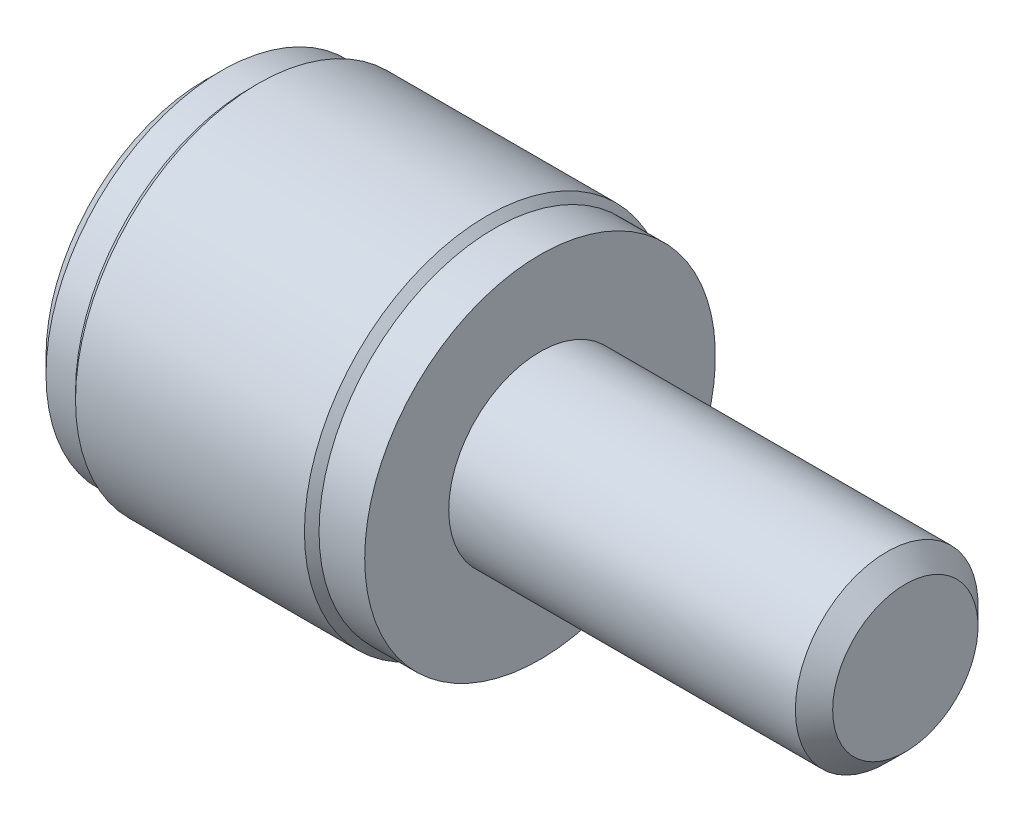
from build123d import *

# Parameters (mm, degrees)
CUT_EXTRUDE1_DEPTH = 1.833333333


with BuildPart() as part:
    # Sketch1 → Revolve1 (revolve)
    with BuildSketch(Plane.XY, mode=Mode.PRIVATE) as revolve1_sk:
        Polygon((-5.5, 0), (-5.5, 2.614834957), (-5.234834957, 2.88), (-4.75, 2.88), (-4.63, 3), (-0.87, 3), (-0.75, 2.88), (0, 2.88), (0, 1.5), (5.6935, 1.5), (6, 1.1935), (6, 0), align=None)
    revolve(revolve1_sk.sketch.rotate(Axis((6, 0, 0), (-1, 0, 0)), 270), axis=Axis((6, 0, 0), (-1, 0, 0)))

    # Sketch2 → Cut-Revolve1 (revolve, cut)
    with BuildSketch(Plane.XY, mode=Mode.PRIVATE) as cut_revolve1_sk:
        Polygon((-5.5, 0), (-5.5, 0.91), (-5.11, 0.52), (-3.05022214, 0.52), (-2.75, 0), align=None)
    revolve(cut_revolve1_sk.sketch.rotate(Axis((-2.75, 0, 0), (-1, 0, 0)), 270), axis=Axis((-2.75, 0, 0), (-1, 0, 0)), mode=Mode.SUBTRACT)

    # Sketch3 → Cut-Extrude1 (cut)
    with BuildSketch(Plane(origin=(-5.5, 0, 0), x_dir=(0, 0, -1), z_dir=(1, 0, 0))):
        Polygon((-0.65, 0.375277675), (-0.65, -0.375277675), (0, -0.75055535), (0.65, -0.375277675), (0.65, 0.375277675), (0, 0.75055535), align=None)
    extrude(amount=CUT_EXTRUDE1_DEPTH, mode=Mode.SUBTRACT)


solid = part.part
